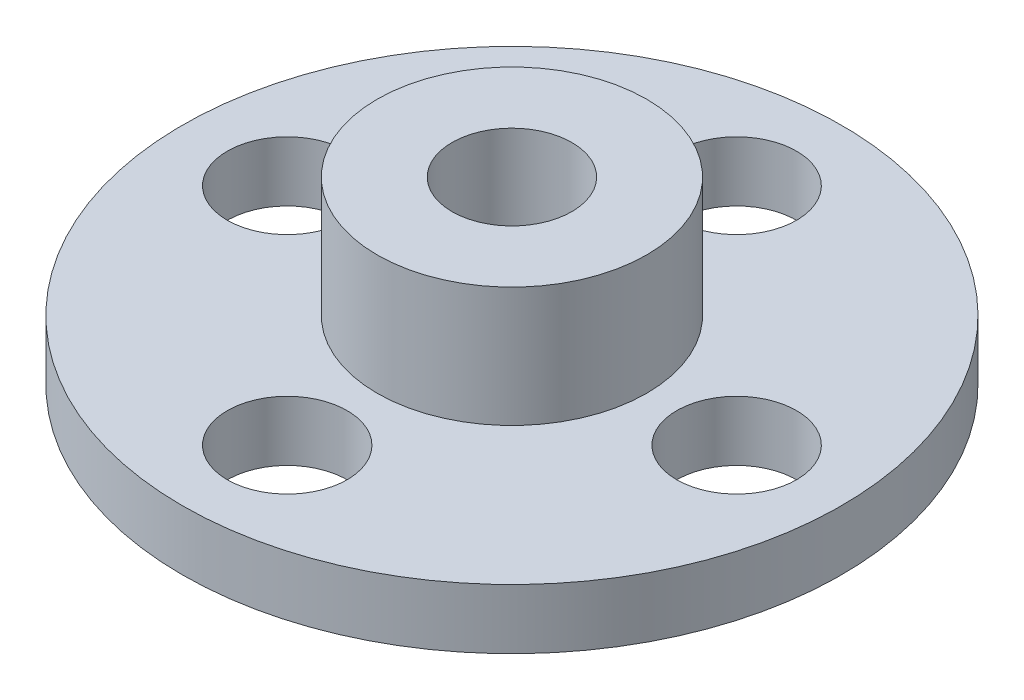
SolidWorks part; units mm, degrees
ref_plane "Front Plane" through (0, 0, 0) normal (0, 0, 1) x (1, 0, 0)
ref_plane "Top Plane" through (0, 0, 0) normal (0, 1, 0) x (1, 0, 0)
ref_plane "Right Plane" through (0, 0, 0) normal (1, 0, 0) x (0, 0, -1)
sketch "Sketch1" plane through (0, 0, 0) normal (0, 1, 0) x (1, 0, 0)
  circle A0 centre (0, 0) radius 11
  circle A1 centre (0, 0) radius 7.5 construction
  circle A2 centre (0, 7.5) radius 2
  circle A3 centre (7.5, 0) radius 2
  circle A4 centre (0, -7.5) radius 2
  circle A5 centre (-7.5, 0) radius 2
  point P15 (0, 0)
  dimension "D1" = 22
  dimension "D2" = 15
  dimension "D3" = 4
  dimension "D4" = 4
extrude "Boss-Extrude1" add sketch "Sketch1" along normal blind 2
sketch "Sketch2" plane through (0, 2, 0) normal (0, 1, 0) x (1, 0, 0)
  circle A0 centre (0, 0) radius 4.5
  dimension "D1" = 9
extrude "Boss-Extrude2" add sketch "Sketch2" along normal blind 4
sketch "Sketch3" plane through (0, 6, 0) normal (0, 1, 0) x (1, 0, 0)
  circle A0 centre (0, 0) radius 2
  dimension "D1" = 4
extrude "Cut-Extrude1" cut sketch "Sketch3" against normal through all both and the other way through all
